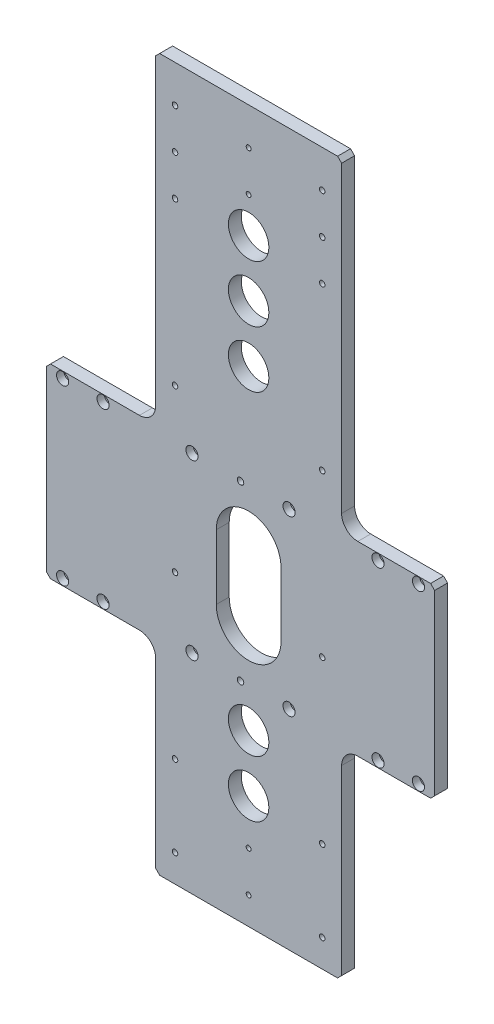
from build123d import *

# Parameters (mm, degrees)
SKETCH_1_W                = 230
SKETCH_1_H                = 400
SKETCH_1_W_2              = 480
SKETCH_1_H_2              = 230
SKETCH_1_H_3              = 250
EXTRUDE_1_DEPTH           = 16
FILLET_1_R                = 20
HOLE_WIZARD_1_D           = 9
HOLE_WIZARD_1_CBORE_D     = 15
HOLE_WIZARD_1_CBORE_DEPTH = 9
MM_1_D                    = 8
HOLE_WIZARD_M8_1_D        = 6.8
HOLE_WIZARD_M8_1_DEPTH    = 22.25
HOLE_WIZARD_M8_1_TIP      = 2.042926105
CHAMFER_2_SIZE            = 5
CHAMFER_3_SIZE            = 5
SKETCH_8_R                = 25
CUT_EXTRUDE_1_DEPTH       = 569.402146372
MM_2_D                    = 6


with BuildPart() as part:
    # 草图1 → 凸台-拉伸1 (new body)
    with BuildSketch(Plane.XY):
        with Locations((10, 315)):
            Rectangle(SKETCH_1_W, SKETCH_1_H)
        Rectangle(SKETCH_1_W_2, SKETCH_1_H_2)
        with Locations((10, -240)):
            Rectangle(SKETCH_1_W, SKETCH_1_H_3)
    extrude(amount=EXTRUDE_1_DEPTH)

    # 圆角1
    fillet_1_edges = [part.edges().sort_by_distance(p)[0] for p in [
        (125, 115, 8),
        (125, -115, 8),
        (-105, -115, 8),
        (-105, 115, 8),
    ]]
    fillet(fillet_1_edges, radius=FILLET_1_R)

    # 打孔尺寸(%根据)内六角圆柱头螺钉的类型1 (through all)
    with Locations(Plane.XY.offset(16)):
        with Locations((60, -107), (220, 107), (-220, -107), (-220, 107), (220, -107), (-170, 107), (-170, -107), (170, 107), (170, -107), (-60, 107), (-60, -107), (60, 107)):
            CounterBoreHole(HOLE_WIZARD_1_D / 2, HOLE_WIZARD_1_CBORE_D / 2, HOLE_WIZARD_1_CBORE_DEPTH)

    # 大小mm 暗销孔1 (through all)
    with Locations(Plane.XY.offset(16)):
        with Locations((0, 107), (0, -107)):
            Hole(MM_1_D / 2)

    # M8 螺纹孔1
    with Locations(Plane.XY.offset(16)):
        with Locations((101, 469), (-81, 469), (-81, 169), (-81, 369), (-81, 419), (-81, -31), (-81, -231), (-81, -331), (101, -331), (101, -231), (101, -31), (101, 419), (101, 369), (101, 169)):
            Hole(HOLE_WIZARD_M8_1_D / 2, depth=HOLE_WIZARD_M8_1_DEPTH)
            with Locations((0, 0, -(HOLE_WIZARD_M8_1_DEPTH + HOLE_WIZARD_M8_1_TIP / 2))):  # 118° drill point
                Cone(0, HOLE_WIZARD_M8_1_D / 2, HOLE_WIZARD_M8_1_TIP, mode=Mode.SUBTRACT)

    # 倒角2
    chamfer_2_edges = [part.edges().sort_by_distance(p)[0] for p in [
        (125, -365, 8),
        (-105, -365, 8),
        (-105, 515, 8),
        (125, 515, 8),
    ]]
    chamfer(chamfer_2_edges, length=CHAMFER_2_SIZE)

    # 倒角3
    chamfer_3_edges = [part.edges().sort_by_distance(p)[0] for p in [
        (240, 115, 8),
        (240, -115, 8),
        (-240, -115, 8),
        (-240, 115, 8),
    ]]
    chamfer(chamfer_3_edges, length=CHAMFER_3_SIZE)

    # 草图8 → 切除-拉伸1 (cut, through all)
    with BuildSketch(Plane.XY.offset(16)):
        with Locations((10, 375)):
            Circle(SKETCH_8_R)
        with Locations((10, 305)):
            Circle(SKETCH_8_R)
        with Locations((10, -155)):
            Circle(SKETCH_8_R)
        with Locations((10, -225)):
            Circle(SKETCH_8_R)
        with Locations((10, 235)):
            Circle(SKETCH_8_R)
        with BuildLine():
            Line((50, 40), (50, -40))
            ThreePointArc((50, -40), (10, -80), (-30, -40))
            Line((-30, -40), (-30, 40))
            ThreePointArc((-30, 40), (10, 80), (50, 40))
        make_face()
    extrude(amount=-CUT_EXTRUDE_1_DEPTH, mode=Mode.SUBTRACT)

    # 大小mm 暗销孔2 (through all)
    with Locations(Plane.XY.offset(16)):
        with Locations((10, -281), (10, 469), (10, 419), (10, -331)):
            Hole(MM_2_D / 2)


solid = part.part
